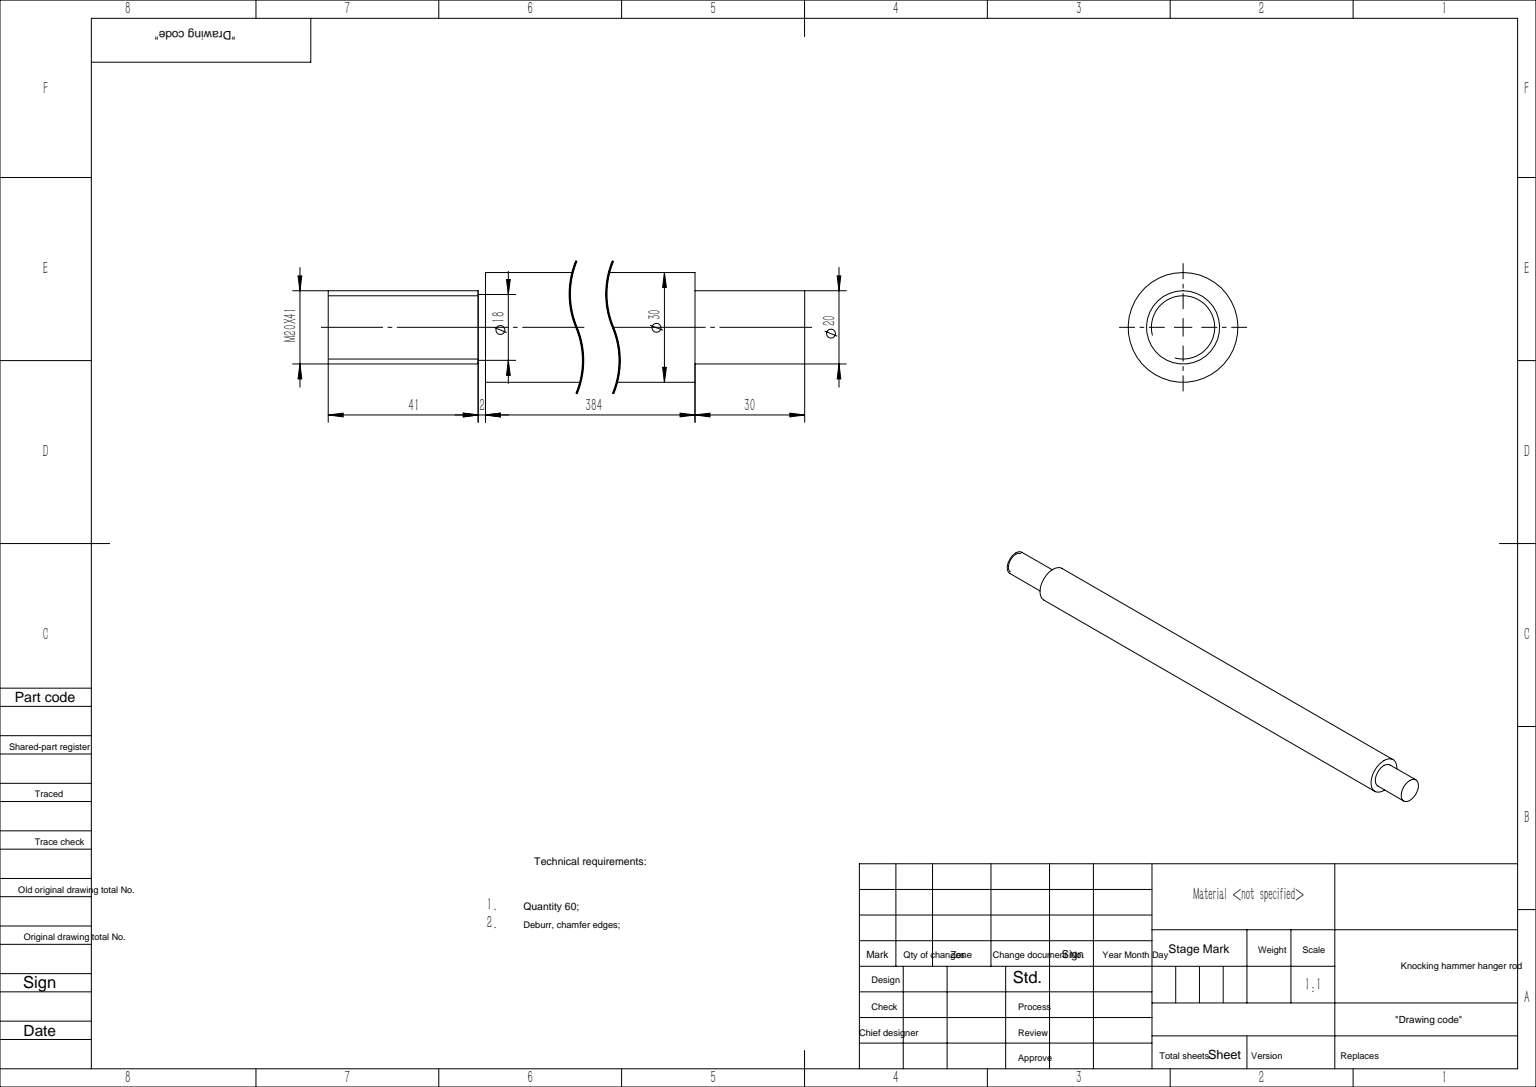
SolidWorks part; units mm, degrees
ref_plane "前视基准面" through (0, 0, 0) normal (0, 0, 1) x (1, 0, 0)
ref_plane "上视基准面" through (0, 0, 0) normal (0, 1, 0) x (1, 0, 0)
ref_plane "右视基准面" through (0, 0, 0) normal (1, 0, 0) x (0, 0, -1)
sketch "草图1" plane through (0, 0, 0) normal (0, 0, 1) x (1, 0, 0)
  line L1 (0, 0) -> (0, 10)
  line L2 (0, 10) -> (43, 10)
  line L3 (43, 10) -> (43, 15)
  line L4 (43, 15) -> (427, 15)
  line L5 (427, 15) -> (427, 10)
  line L6 (427, 10) -> (457, 10)
  line L7 (457, 10) -> (457, 0)
  line L8 (457, 0) -> (0, 0)
  dimension "D1" = 10
  dimension "D2" = 10
  dimension "D3" = 15
  dimension "D4" = 43
  dimension "D5" = 384
  dimension "D6" = 30
revolve "旋转1" add sketch "草图1" angle 360 about L8
cosmetic thread "装饰螺纹线1" parameters "D1"=41, "D2"=17.294
sketch "草图2" plane through (43, 0, 0) normal (-1, 0, 0) x (0, 0, 1)
  circle A0 centre (0, 0) radius 10 construction
  circle A1 centre (0, 0) radius 10
  circle A2 centre (0, 0) radius 9
  dimension "D1" = 1
extrude "切除-拉伸1" cut sketch "草图2" along normal blind 2
